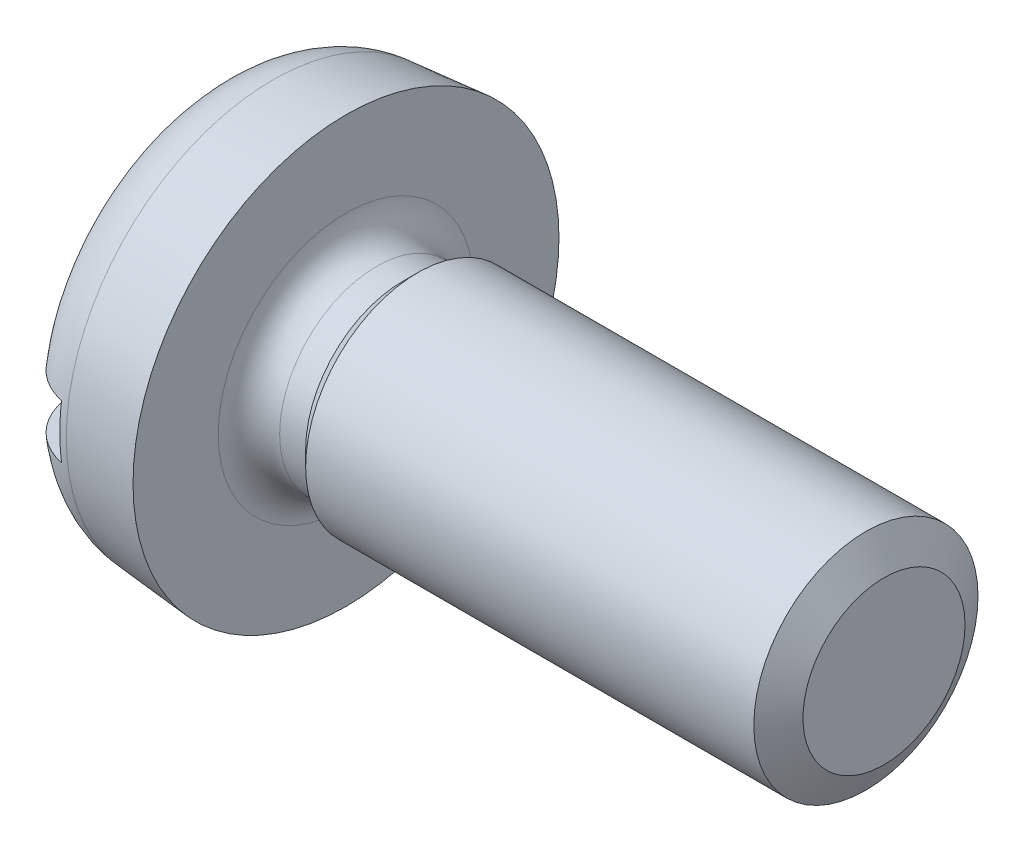
SolidWorks part; units mm, degrees
revolve "Boss-Revolve" add sketch "Sketch3" angle 360 about L0
sketch "Sketch3" plane through (0, 0, 0) normal (0, 0, 1) x (1, 0, 0)
  line L0 (-2.477, 0) -> (6.7868, 0) construction
  line L1 (0, 0) -> (15, 0)
  line L2 (15, 0) -> (15, 2.5)
  line L3 (15, 2.5) -> (4.6, 2.5)
  line L4 (3, 2.85) -> (3, 4.75)
  line L5 (4.6, 2.5) -> (4.265, 2.165)
  line L6 (4.265, 2.165) -> (3.685, 2.165)
  line L7 (3, 4.75) -> (1.3693, 4.6073)
  line L9 (0, 3.113) -> (0, 0)
  arc A0 (3.685, 2.165) -> (3, 2.85) centre (3.685, 2.85) cw
  arc A1 (1.3693, 4.6073) -> (0, 3.113) centre (1.5, 3.113) ccw
cosmetic thread "Cosmetic Thread1" parameters "D1"=10.4, "D2"=4.33
material "Grade 4.8"
ref_plane "Front" through (0, 0, 0) normal (0, 0, 1) x (1, 0, 0)
ref_plane "Top" through (0, 0, 0) normal (0, 1, 0) x (1, 0, 0)
ref_plane "Right" through (0, 0, 0) normal (1, 0, 0) x (0, 0, -1)
sketch "Dimension Sketch" plane through (0, 0, 0) normal (0, 0, 1) x (1, 0, 0)
  line L0 (0, 0) -> (12, 0)
  line L1 (0, 0) -> (0, 9.5)
  line L2 (12, 0) -> (12, 5.7)
  point P5 (11.2, 0)
  point P6 (3, 0)
  point P7 (1.2, 0)
  point P8 (1.6, 0)
  point P9 (12, 0.2)
  point P10 (10.5, 0)
  point P11 (0, 1.2)
  point P12 (12, 5)
sketch "Sketch4" plane through (0, 0, 0) normal (0, 0, 1) x (1, 0, 0)
  line L0 (0, 3.113) -> (0, -3.113) construction
  line L1 (0, 0.6) -> (1.2, 0.6)
  line L2 (0, 0.6) -> (0, -0.6)
  line L3 (0, -0.6) -> (1.2, -0.6)
  line L4 (1.2, 0.6) -> (1.2, -0.6)
  point P6 (0, 0)
extrude "Cut-Extrude1" cut sketch "Sketch4" against normal mid plane 100
sketch "Sketch5" plane through (0, 0, 0) normal (0, 0, 1) x (1, 0, 0)
  line L0 (14.5957, 2.5) -> (15.3957, 2.5)
  line L1 (15.3957, 2.5) -> (15, 1.8072)
  line L2 (15, 1.8072) -> (14.5957, 2.5)
  line L3 (15, 2.5) -> (4.6, 2.5) construction
  line L4 (15, -2.5) -> (15, 2.5) construction
  line L5 (6.175, 0) -> (-0.2582, 0) construction
  line L6 (-2.477, 0) -> (6.7868, 0) construction
revolve "Cut-Revolve1" cut sketch "Sketch5" angle 360 about L5
pattern_linear "LPattern1" [suppressed] count 14 spacing 0.8 along (1, 0, 0)
equation "\"l@Sketch3\" = \"l@Dimension Sketch\""
equation "\"dk@Sketch3\"=\"dk@Dimension Sketch\""
equation "\"da@Sketch3\" = \"da@Dimension Sketch\""
equation "\"D3@Sketch3\" = \"d@Dimension Sketch\"*0.866"
equation "\"D4@Sketch3\" = \"l@Dimension Sketch\"-\"a@Dimension Sketch\""
equation "\"d@Sketch3\" = \"d@Dimension Sketch\""
equation "\"D2@Cosmetic Thread1\" = \"d@Dimension Sketch\"*0.866"
equation "\"D1@Cosmetic Thread1\" = \"l@Dimension Sketch\"-\"a@Dimension Sketch\""
equation "\"n@Sketch4\" = \"n@Dimension Sketch\""
equation "\"t@Sketch4\" = \"t@Dimension Sketch\""
equation "\"P@Sketch5\" = \"P@Dimension Sketch\""
equation "\"D1@Sketch5\" = \"P@Sketch5\"*0.866"
equation "\"D3@LPattern1\" = \"P@Dimension Sketch\""
equation "\"D1@LPattern1\" = (\"l@Dimension Sketch\"-\"a@Dimension Sketch\")/\"P@Dimension Sketch\"+1"
equation "\"k@Sketch3\"=\"k@Dimension Sketch\""
equation "\"D5@Sketch3\"=\"rf@Dimension Sketch\""
